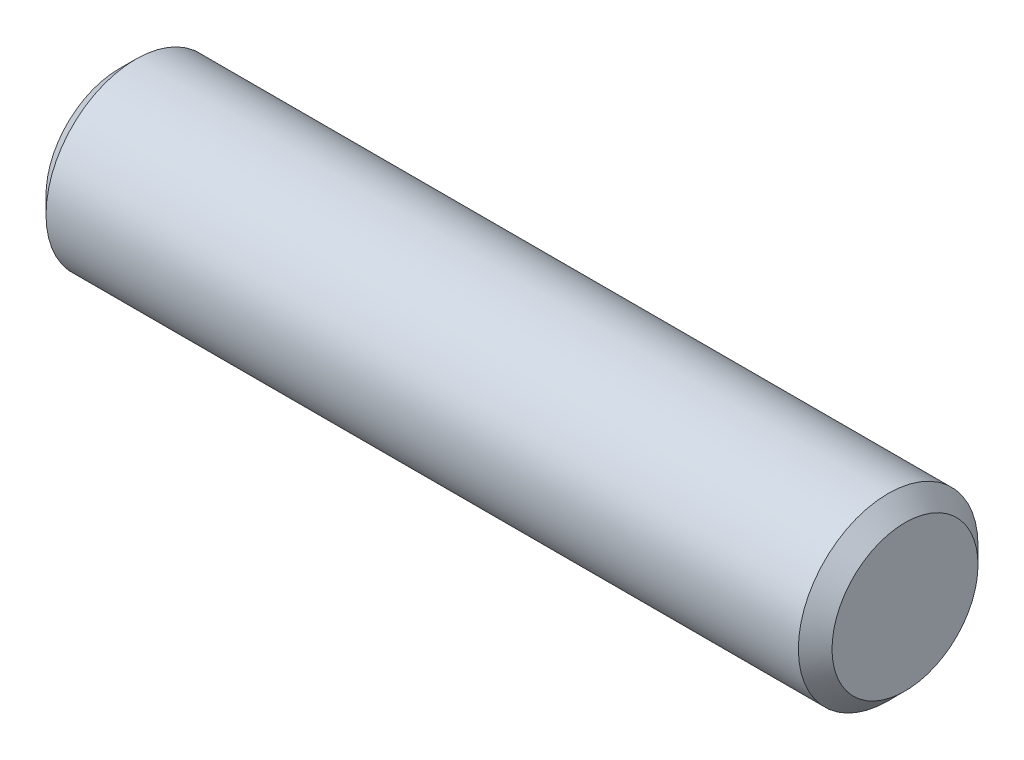
SolidWorks part; units mm, degrees
ref_plane "Front Plane" through (0, 0, 0) normal (0, 0, 1) x (1, 0, 0)
ref_plane "Top Plane" through (0, 0, 0) normal (0, 1, 0) x (1, 0, 0)
ref_plane "Right Plane" through (0, 0, 0) normal (1, 0, 0) x (0, 0, -1)
other "Configuration Table"
sketch "Sketch1" plane through (0, 0, 0) normal (0, 0, 1) x (1, 0, 0)
  line L0 (-70, 14.5) -> (-70, 8)
  line L1 (-70, 8) -> (0, 8)
  line L2 (0, 8) -> (0, 14.5)
  line L3 (0, 14.5) -> (-1.5, 16)
  line L4 (-1.5, 16) -> (-68.5, 16)
  line L5 (-68.5, 16) -> (-70, 14.5)
  line L6 (-70, 8) -> (0, 8) construction
revolve "Revolve1" add sketch "Sketch1" angle 360 about L6
